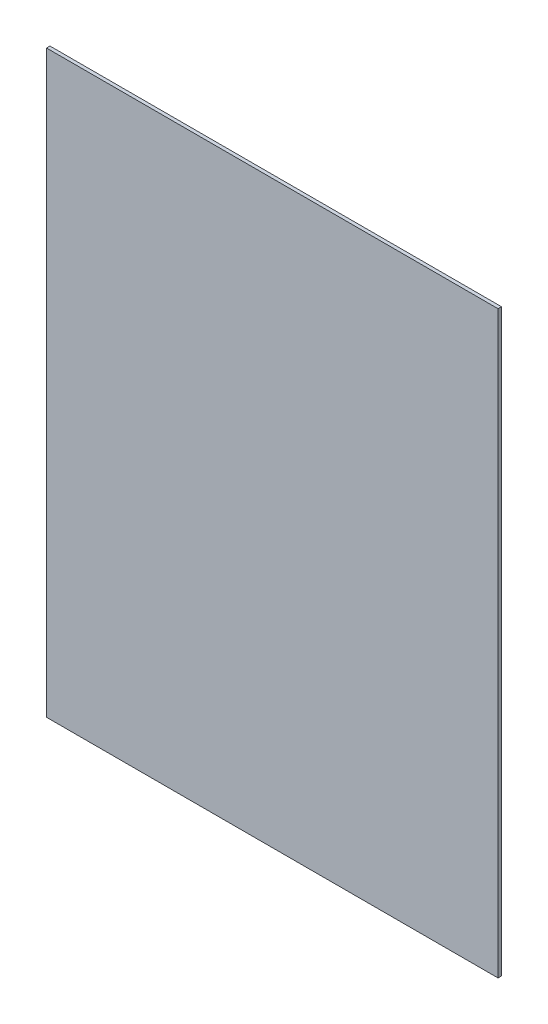
SolidWorks part; units mm, degrees
material "PMMA(有机玻璃)"
ref_plane "前视" through (0, 0, 0) normal (0, 0, 1) x (1, 0, 0)
ref_plane "上视" through (0, 0, 0) normal (0, 1, 0) x (1, 0, 0)
ref_plane "右视" through (0, 0, 0) normal (1, 0, 0) x (0, 0, -1)
sketch "草图1" plane through (0, 0, 0) normal (0, 0, 1) x (1, 0, 0)
  line L1 (-328, 421) -> (328, 421)
  line L2 (-328, 421) -> (-328, -421)
  line L3 (-328, -421) -> (328, -421)
  line L4 (328, 421) -> (328, -421)
  line L5 (-328, 421) -> (328, -421) construction
  line L6 (-328, -421) -> (328, 421) construction
  point P0 (0, 0)
  dimension "D1" = 842
  dimension "D2" = 656
extrude "凸台-拉伸1" add sketch "草图1" along normal blind 5
hole_wizard "M5 间隙孔1" positions "草图3" profile "草图2" hole size "M5" standard "GB"
sketch "草图3" plane through (0, 0, 5) normal (0, 0, 1) x (1, 0, 0)
  line L0 (-427.5, 273) -> (-427.5, -273) construction
  line L1 (-427.5, -273) -> (427.5, -273) construction
  line L2 (0, 273) -> (0, -273) construction
  line L3 (427.5, 273) -> (-427.5, 273) construction
  line L5 (-427.5, 0) -> (427.5, 0) construction
  line L6 (427.5, -273) -> (427.5, 273) construction
  point P0 (-375, -261)
  point P46 (415.5, 250)
  point P48 (-415.5, 250)
  point P58 (-125, -261)
  point P59 (125, -261)
  point P61 (-125, 261)
  point P62 (125, 261)
  point P64 (-375, 261)
  point P88 (375, -261)
  point P89 (375, 261)
  point P108 (415.5, 0)
  point P109 (-415.5, 0)
  point P110 (415.5, -250)
  point P111 (-415.5, -250)
  dimension "D1" = 12
  dimension "D2" = 12
  dimension "D5" = 3
  dimension "D3" = 12
  dimension "D6" = 4
  dimension "D4" = 2
sketch "草图2" plane through (-375, -261, 5) normal (1, 0, 0) x (0, -1, 0)
  line L0 (0, 0) -> (0, 5)
  line L1 (0, 5) -> (2.75, 5)
  line L2 (2.75, 5) -> (2.75, 0)
  line L5 (2.75, 0) -> (0, 0)
  line L11 (0, -6.35) -> (0, 107.95) construction
  dimension "通孔孔直径" = 5.5
  dimension "通孔孔深度" = 5
